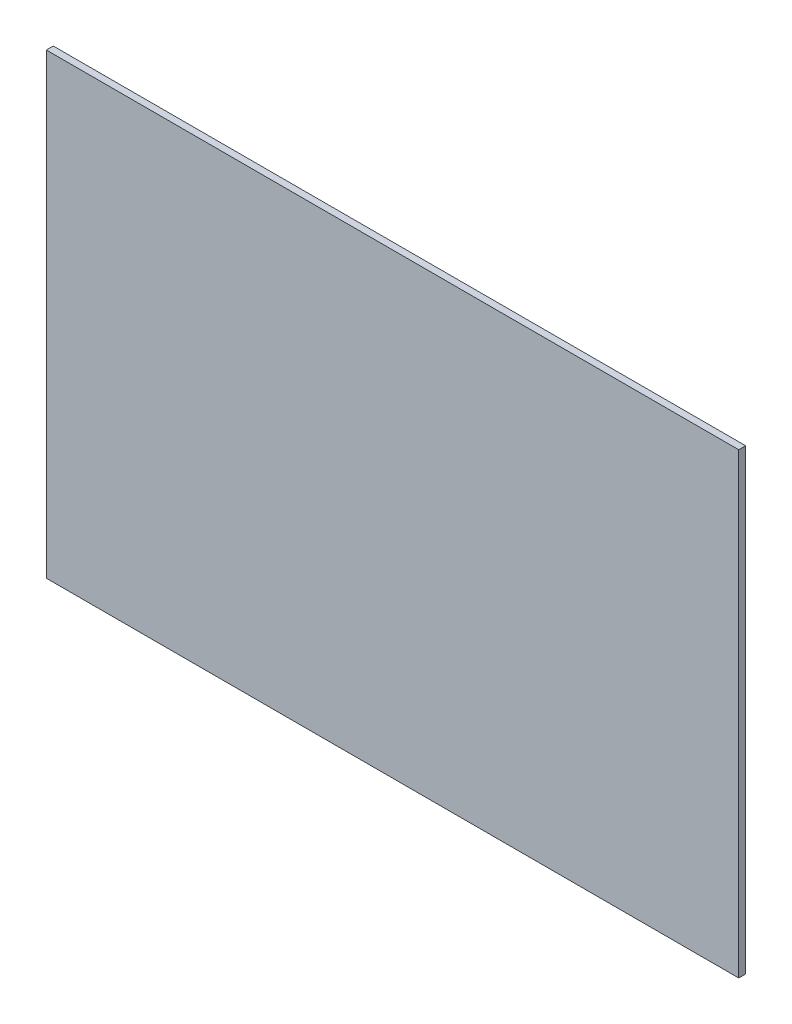
from build123d import *

# Parameters (mm, degrees)
SKETCH_1_W      = 1400
SKETCH_1_H      = 925
EXTRUDE_1_DEPTH = 14


with BuildPart() as part:
    # 草图1 → 凸台-拉伸1 (new body)
    with BuildSketch(Plane.XY):
        with Locations((-75, 362.5)):
            Rectangle(SKETCH_1_W, SKETCH_1_H)
    extrude(amount=EXTRUDE_1_DEPTH)


solid = part.part
